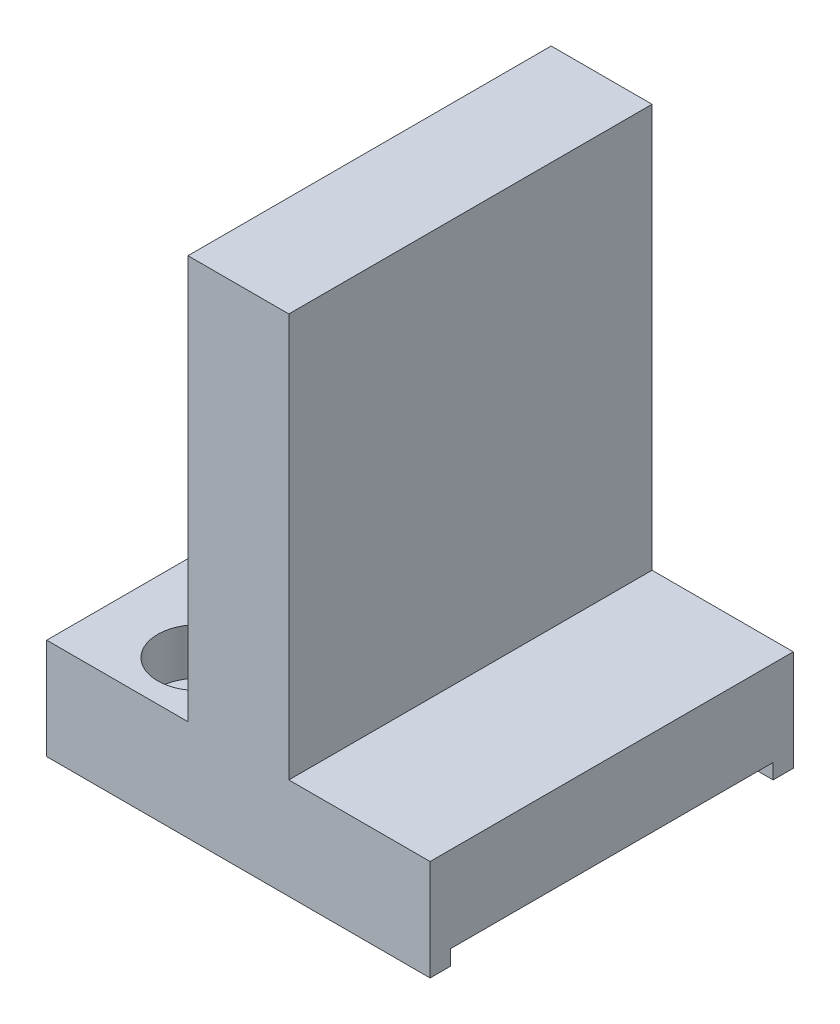
from build123d import *

# Parameters (mm, degrees)
EXTRUDE_1_DEPTH           = 18
SKETCH_2_W                = 38
SKETCH_2_H                = 32
CUT_EXTRUDE_1_DEPTH       = 1.5
HOLE_WIZARD_1_D           = 4.5
HOLE_WIZARD_1_CBORE_D     = 8
HOLE_WIZARD_1_CBORE_DEPTH = 4.6


with BuildPart() as part:
    # 草图1 → 凸台-拉伸1 (new, symmetric)
    with BuildSketch(Plane.XY):
        Polygon((0, 0), (-19, 0), (-19, 10), (-5, 10), (-5, 50), (5, 50), (5, 10), (19, 10), (19, 0), align=None)
    extrude(amount=EXTRUDE_1_DEPTH, both=True)

    # 草图2 → 切除-拉伸1 (cut)
    with BuildSketch(Plane.XZ):
        Rectangle(SKETCH_2_W, SKETCH_2_H)
    extrude(amount=-CUT_EXTRUDE_1_DEPTH, mode=Mode.SUBTRACT)

    # 打孔尺寸(%根据)内六角圆柱头螺钉的类型1 (through all)
    with Locations(Plane(origin=(-10, 10, 12), x_dir=(0, 0, 1), z_dir=(0, 1, 0))):
        with Locations((0, 0)):
            CounterBoreHole(HOLE_WIZARD_1_D / 2, HOLE_WIZARD_1_CBORE_D / 2, HOLE_WIZARD_1_CBORE_DEPTH)


solid = part.part
